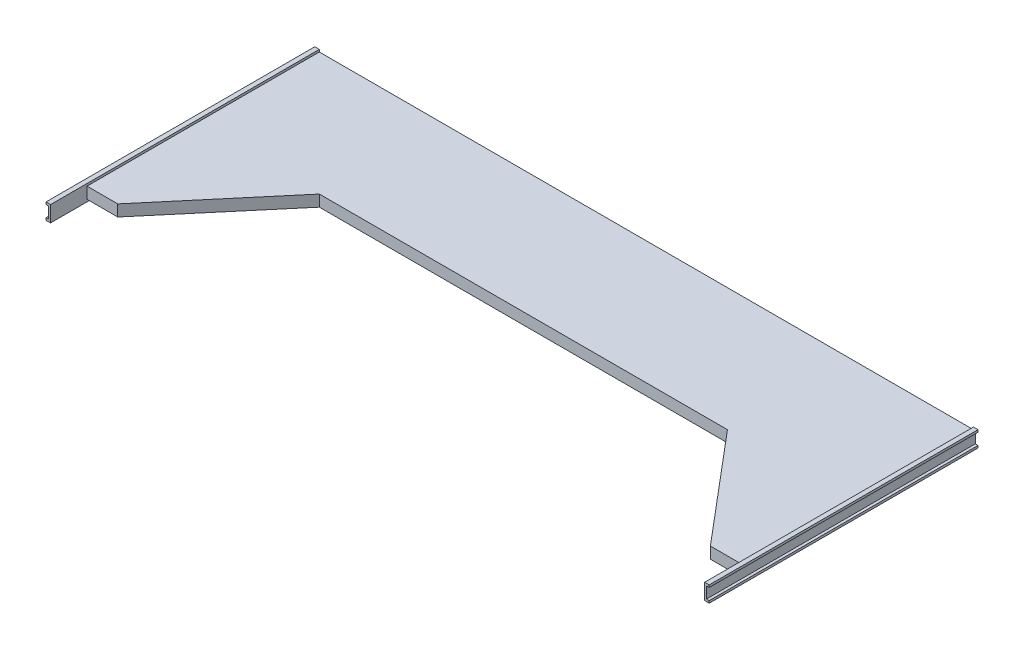
SolidWorks part; units mm, degrees
ref_plane "Front Plane" through (0, 0, 0) normal (0, 0, 1) x (1, 0, 0)
ref_plane "Top Plane" through (0, 0, 0) normal (0, 1, 0) x (1, 0, 0)
ref_plane "Right Plane" through (0, 0, 0) normal (1, 0, 0) x (0, 0, -1)
sketch "Sketch1" plane through (0, 0, 0) normal (0, 0, 1) x (1, 0, 0)
  line L0 (10, 25) -> (10, 30)
  line L1 (10, 0) -> (1446, 0)
  line L2 (0, 30) -> (0, 25)
  line L3 (10, 25) -> (1446, 25)
  line L4 (1446, 0) -> (1446, 25) construction
  line L5 (10, 30) -> (0, 30)
  line L6 (0, 25) -> (5, 25)
  line L7 (5, 0) -> (3209.1429, 0) construction
  line L8 (10, -5) -> (10, 0)
  line L9 (10, 25) -> (10, 0) construction
  line L10 (5, 25) -> (5, 0)
  line L11 (5, 0) -> (0, 0)
  line L12 (0, 0) -> (0, -5)
  line L13 (0, -5) -> (10, -5)
  line L14 (1446, 30) -> (1446, 25)
  line L15 (1446, 30) -> (1456, 30)
  line L16 (1456, 30) -> (1456, 25)
  line L17 (1456, 25) -> (1450, 25)
  line L18 (1450, 25) -> (1450, 0)
  line L19 (1450, 0) -> (1456, 0)
  line L20 (1456, 0) -> (1456, -5)
  line L21 (1456, -5) -> (1446, -5)
  line L22 (1446, -5) -> (1446, 0)
  dimension "D1" = 5
  dimension "D2" = 5
  dimension "D3" = 10
  dimension "D4" = 5
  dimension "D5" = 25
  dimension "D6" = 5
  dimension "D7" = 10
  dimension "D8" = 6
  dimension "D9" = 5
  dimension "D10" = 1456
extrude "Boss-Extrude1" add sketch "Sketch1" along normal blind 590
sketch "Sketch2" plane through (0, 25, 0) normal (0, 1, 0) x (1, 0, 0)
  line L0 (10, -590) -> (305, -295) construction
  line L1 (305, -295) -> (1151, -295) construction
  line L2 (1151, -295) -> (1446, -590) construction
  line L3 (1446, -590) -> (10, -590) construction
  line L5 (10, -590) -> (10, 0) construction
  line L6 (10, -590) -> (1446, -590)
  line L7 (77.5, -510) -> (280, -270)
  line L8 (280, -270) -> (1176, -270)
  line L9 (1176, -270) -> (1378.5, -510)
  line L10 (10, -510) -> (77.5, -510)
  line L11 (1378.5, -510) -> (1446, -510)
  line L12 (1446, -590) -> (1446, 0) construction
  line L13 (1446, -510) -> (1446, -590)
  line L14 (10, -510) -> (10, -590)
  line L15 (77.5, -510) -> (10, -590) construction
  line L16 (1378.5, -510) -> (1446, -590) construction
  dimension "D1" = 295
  dimension "D2" = 295
  dimension "D3" = 25
  dimension "D4" = 25
  dimension "D5" = 25
  dimension "D6" = 80
extrude "Cut-Extrude1" cut sketch "Sketch2" against normal up to next
